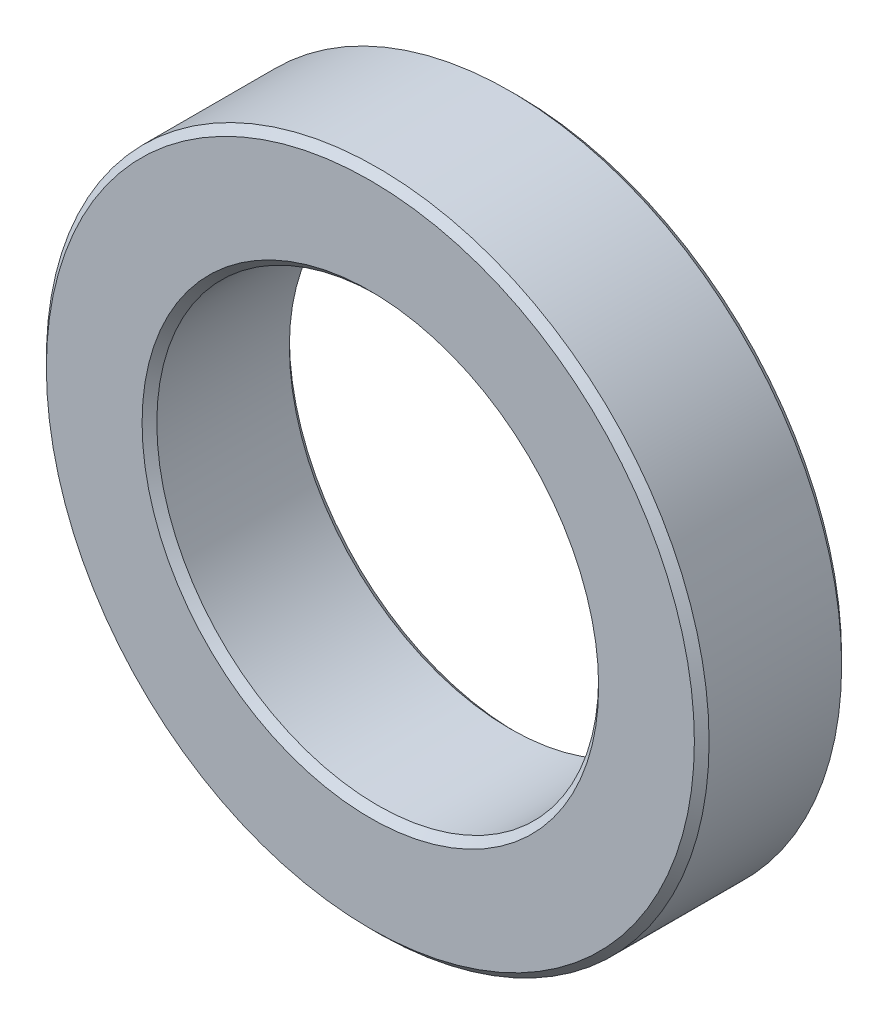
from build123d import *

# Parameters (mm, degrees)
SKETCH1_R           = 22.5
SKETCH1_R_2         = 15
BOSS_EXTRUDE1_DEPTH = 10
CHAMFER1_SIZE       = 0.5


with BuildPart() as part:
    # Sketch1 → Boss-Extrude1 (new body)
    with BuildSketch(Plane.XY):
        Circle(SKETCH1_R)
        Circle(SKETCH1_R_2, mode=Mode.SUBTRACT)
    extrude(amount=BOSS_EXTRUDE1_DEPTH)

    # Chamfer1
    chamfer1_edges = [part.edges().sort_by_distance(p)[0] for p in [
        (-22.5, 0, 0),
        (-22.5, 0, 10),
        (-15, 0, 0),
        (-15, 0, 10),
    ]]
    chamfer(chamfer1_edges, length=CHAMFER1_SIZE)


solid = part.part
